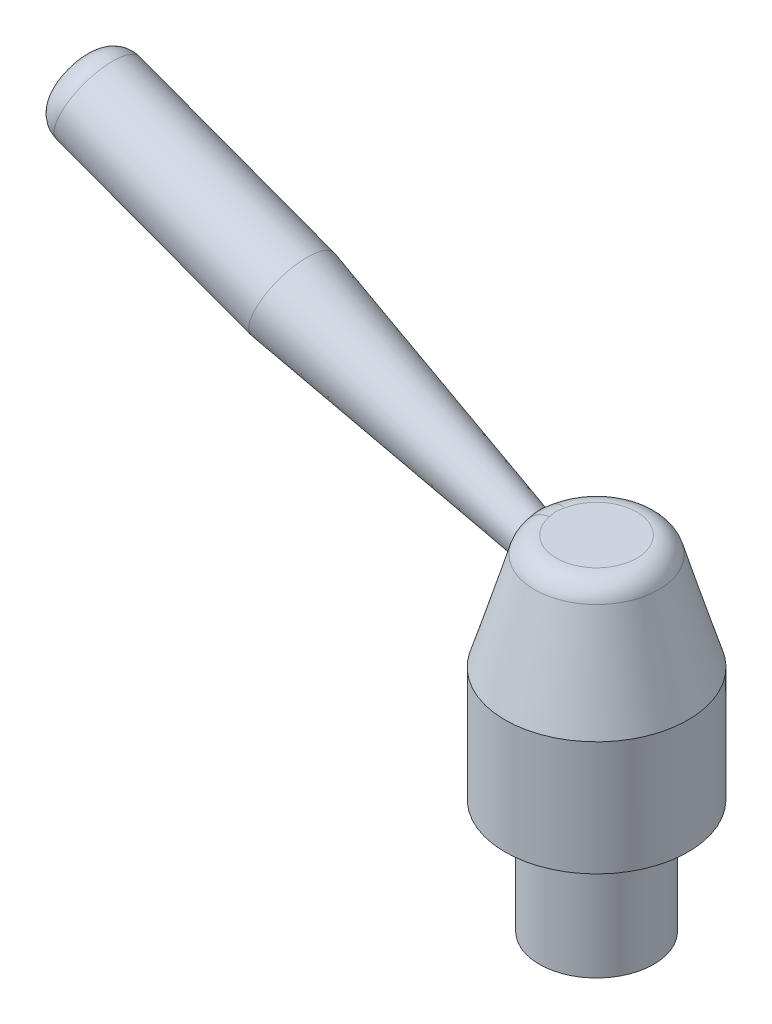
SolidWorks part; units mm, degrees
ref_plane "Front Plane" through (0, 0, 0) normal (0, 0, 1) x (1, 0, 0)
ref_plane "Top Plane" through (0, 0, 0) normal (0, 1, 0) x (1, 0, 0)
ref_plane "Right Plane" through (0, 0, 0) normal (1, 0, 0) x (0, 0, -1)
sketch "Sketch2" plane through (0, 0, 0) normal (0, 0, 1) x (1, 0, 0)
  line L0 (0, 0) -> (0, 10)
  line L2 (-8, 10) -> (-8, 0)
  line L3 (-8, 0) -> (0, 0)
  line L4 (-8, 10) -> (-5, 20)
  line L5 (-5, 20) -> (0, 20)
  line L6 (0, 20) -> (0, 10)
  dimension "D1" = 8
  dimension "D2" = 10
  dimension "D3" = 20
  dimension "D4" = 5
revolve "Revolve1" add sketch "Sketch2" angle 360 about L6
sketch "Sketch3" plane through (0, 0, 0) normal (0, 0, 1) x (1, 0, 0)
  line L0 (-3.6463, 16.4233) -> (-39.9415, 29.9516) construction
  line L1 (-45.4573, 32.0074) -> (-46.7211, 28.6168)
  line L2 (-46.7211, 28.6168) -> (-27.8445, 21.581)
  line L3 (-27.8445, 21.581) -> (-4.1924, 14.9582)
  line L4 (-4.1924, 14.9582) -> (-3.6463, 16.4233)
  line L5 (-3.6463, 16.4233) -> (-45.4573, 32.0074)
revolve "Revolve2" add sketch "Sketch3" angle 360 about L0
sketch "Sketch4" plane through (0, 0, 0) normal (0, -1, 0) x (1, 0, 0)
  circle A0 centre (0, 0) radius 5
extrude "Boss-Extrude1" add sketch "Sketch4" along normal blind 10
fillet "Fillet1" radius 2 2 edges at (-5, 20, 0) (-44.1935, 35.398, 0)
